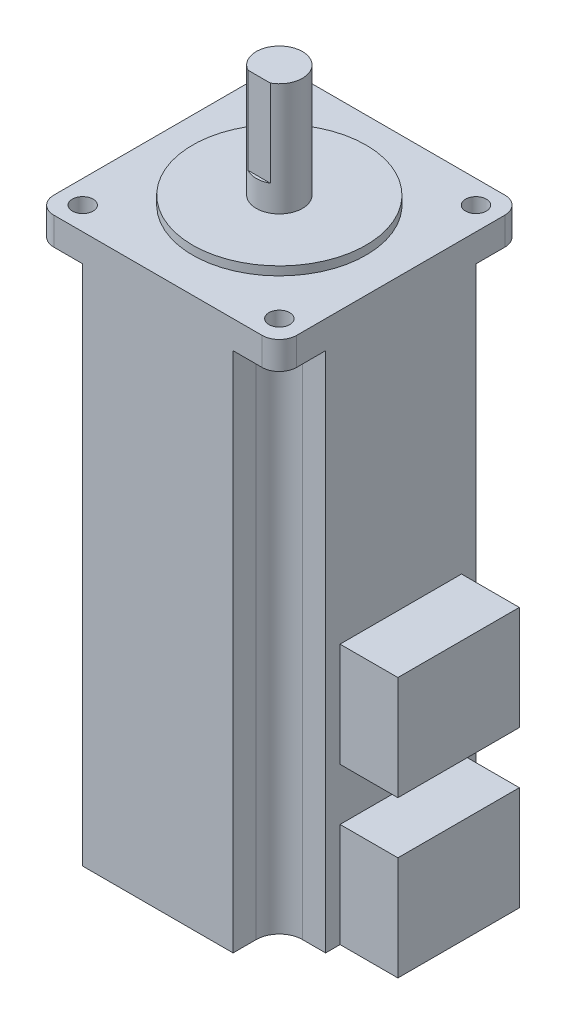
from build123d import *

# Parameters (mm, degrees)
SKETCH1_W           = 42
SKETCH1_H           = 42
BOSS_EXTRUDE1_DEPTH = 95
SKETCH2_W           = 8
SKETCH2_H           = 8
CUT_EXTRUDE1_DEPTH  = 90.2
SKETCH3_R           = 1.8
CUT_EXTRUDE2_DEPTH  = 4.8
FILLET1_R           = 4
SKETCH4_R           = 15
BOSS_EXTRUDE2_DEPTH = 1.5
SKETCH5_R           = 4
BOSS_EXTRUDE3_DEPTH = 21
FILLET2_R           = 3
SKETCH8_W           = 21
SKETCH8_H           = 18
BOSS_EXTRUDE5_DEPTH = 10
SKETCH9_W           = 13.716177762
SKETCH9_H           = 4.011335006
CUT_EXTRUDE3_DEPTH  = 15


with BuildPart() as part:
    # Sketch1 → Boss-Extrude1 (new body)
    with BuildSketch(Plane(origin=(0, 0, 0), x_dir=(1, 0, 0), z_dir=(0, 1, 0))):
        Rectangle(SKETCH1_W, SKETCH1_H)
    extrude(amount=BOSS_EXTRUDE1_DEPTH)

    # Sketch2 → Cut-Extrude1 (cut)
    with BuildSketch(Plane.XZ):
        with Locations((-17, 17)):
            Rectangle(SKETCH2_W, SKETCH2_H)
        with Locations((17, 17)):
            Rectangle(SKETCH2_W, SKETCH2_H)
        with Locations((-17, -17)):
            Rectangle(SKETCH2_W, SKETCH2_H)
        with Locations((17, -17)):
            Rectangle(SKETCH2_W, SKETCH2_H)
    extrude(amount=-CUT_EXTRUDE1_DEPTH, mode=Mode.SUBTRACT)

    # Sketch3 → Cut-Extrude2 (cut)
    with BuildSketch(Plane(origin=(0, 95, 0), x_dir=(1, 0, 0), z_dir=(0, 1, 0))):
        with Locations(Location((-17, 17, 0), (0, 0, 270))):
            Circle(SKETCH3_R)
        with Locations(Location((17, 17, 0), (0, 0, 270))):
            Circle(SKETCH3_R)
        with Locations(Location((-17, -17, 0), (0, 0, 270))):
            Circle(SKETCH3_R)
        with Locations(Location((17, -17, 0), (0, 0, 270))):
            Circle(SKETCH3_R)
    extrude(amount=-CUT_EXTRUDE2_DEPTH, mode=Mode.SUBTRACT)

    # Fillet1
    fillet1_edges = [part.edges().sort_by_distance(p)[0] for p in [
        (-13, 45.1, 13),
        (13, 45.1, 13),
        (-13, 45.1, -13),
        (13, 45.1, -13),
    ]]
    fillet(fillet1_edges, radius=FILLET1_R)

    # Sketch4 → Boss-Extrude2 (add)
    with BuildSketch(Plane(origin=(0, 95, 0), x_dir=(1, 0, 0), z_dir=(0, 1, 0))):
        with Locations(Location((0, 0, 0), (0, 0, 90))):
            Circle(SKETCH4_R)
    extrude(amount=BOSS_EXTRUDE2_DEPTH)

    # Sketch5 → Boss-Extrude3 (add)
    with BuildSketch(Plane(origin=(0, 95, 0), x_dir=(1, 0, 0), z_dir=(0, 1, 0))):
        with Locations(Location((0, 0, 0), (0, 0, 90))):
            Circle(SKETCH5_R)
    extrude(amount=BOSS_EXTRUDE3_DEPTH)

    # Fillet2
    fillet2_edges = [part.edges().sort_by_distance(p)[0] for p in [
        (21, 92.6, 21),
        (-21, 92.6, 21),
        (-21, 92.6, -21),
        (21, 92.6, -21),
    ]]
    fillet(fillet2_edges, radius=FILLET2_R)

    # Sketch8 → Boss-Extrude5 (add)
    with BuildSketch(Plane(origin=(21, 0, 0), x_dir=(0, 0, -1), z_dir=(1, 0, 0))):
        with Locations((0, 9)):
            Rectangle(SKETCH8_W, SKETCH8_H)
        with Locations((0, 36)):
            Rectangle(SKETCH8_W, SKETCH8_H)
    extrude(amount=BOSS_EXTRUDE5_DEPTH)

    # Sketch9 → Cut-Extrude3 (cut)
    with BuildSketch(Plane(origin=(0, 116, 0), x_dir=(1, 0, 0), z_dir=(0, 1, 0))):
        with Locations((-1.407114482, -5.505667503)):
            Rectangle(SKETCH9_W, SKETCH9_H)
    extrude(amount=-CUT_EXTRUDE3_DEPTH, mode=Mode.SUBTRACT)


solid = part.part
